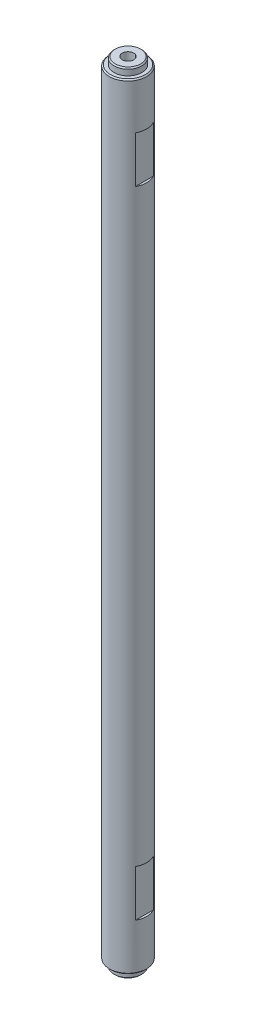
SolidWorks part; units mm, degrees
material "SUJ2"
ref_plane "Front Plane" through (0, 0, 0) normal (0, 0, 1) x (1, 0, 0)
ref_plane "Top Plane" through (0, 0, 0) normal (0, 1, 0) x (1, 0, 0)
ref_plane "Right Plane" through (0, 0, 0) normal (1, 0, 0) x (0, 0, -1)
sketch "Sketch1" plane through (0, 0, 0) normal (0, 1, 0) x (1, 0, 0)
  circle A0 centre (0, 0) radius 8
  dimension "D1" = 16
extrude "Boss-Extrude1" add sketch "Sketch1" along normal mid plane 333
sketch "Sketch2" plane through (0, -166.5, 0) normal (0, -1, 0) x (1, 0, 0)
  circle A0 centre (0, 0) radius 6
  dimension "D1" = 12
extrude "Boss-Extrude2" add sketch "Sketch2" along normal blind 3
chamfer "Chamfer1" distance 0.5 angle 45 2 edges at (0, -169.5, -6) (0, -166.5, 8)
sketch "Sketch3" plane through (0, -166.5, 0) normal (0, -1, 0) x (1, 0, 0)
  line L0 (0, 0) -> (0, 1.7784) construction
  line L1 (-7, 3.873) -> (-7, -3.873)
  line L2 (7, 3.873) -> (7, -3.873)
  circle A0 centre (0, 0) radius 8 construction
  arc A1 (-7, 3.873) -> (-7, -3.873) centre (0, 0) ccw
  arc A2 (7, -3.873) -> (7, 3.873) centre (0, 0) ccw
  dimension "D1" = 14
extrude "Cut-Extrude2" cut sketch "Sketch3" against normal blind 20 from offset 20 offset against normal yes
hole_wizard "M6 Tapped Hole1" positions "Sketch5" profile "Sketch4" tap size "M6" standard "ISO"
sketch "Sketch5" plane through (0, -169.5, 0) normal (0, -1, 0) x (1, 0, 0)
  point P1 (0, 0)
sketch "Sketch4" plane through (0, -169.5, 0) normal (1, 0, 0) x (0, 0, -1)
  line L0 (0, 0) -> (0, 18.5022)
  line L1 (0, 18.5022) -> (2.5, 17)
  line L2 (2.5, 17) -> (2.5, 0)
  line L5 (2.5, 0) -> (0, 0)
  line L10 (0, 18.5022) -> (-2.5, 17) construction
  line L11 (0, -6.35) -> (0, 107.95) construction
  dimension "螺纹孔钻头直径" = 5
  dimension "螺纹孔钻头深度" = 17
  dimension "导头角度" = 118
cosmetic thread "Cosmetic Thread1" parameters "D1"=12, "D2"=6
chamfer "Chamfer2" distance 0.5 angle 45 1 edges at (0, 166.5, 8)
sketch "Sketch6" plane through (0, 166.5, 0) normal (0, 1, 0) x (1, 0, 0)
  circle A0 centre (0, 0) radius 6
  dimension "D1" = 12
extrude "Boss-Extrude3" add sketch "Sketch6" along normal blind 3
chamfer "Chamfer3" distance 0.5 angle 45 1 edges at (0, 169.5, 6)
hole_wizard "M6 Tapped Hole2" positions "Sketch8" profile "Sketch7" tap size "M6" standard "ISO"
sketch "Sketch8" plane through (0, 169.5, 0) normal (0, 1, 0) x (-1, 0, 0)
  point P1 (0, 0)
sketch "Sketch7" plane through (0, 169.5, 0) normal (1, 0, 0) x (0, 0, 1)
  line L0 (0, 0) -> (0, 18.5022)
  line L1 (0, 18.5022) -> (2.5, 17)
  line L2 (2.5, 17) -> (2.5, 0)
  line L5 (2.5, 0) -> (0, 0)
  line L10 (0, 18.5022) -> (-2.5, 17) construction
  line L11 (0, -6.35) -> (0, 107.95) construction
  dimension "螺纹孔钻头直径" = 5
  dimension "螺纹孔钻头深度" = 17
  dimension "导头角度" = 118
cosmetic thread "Cosmetic Thread2" parameters "D1"=12, "D2"=6
mirror "Mirror1" about plane through (0, 0, 0) normal (0, 1, 0) of "Cut-Extrude2"
